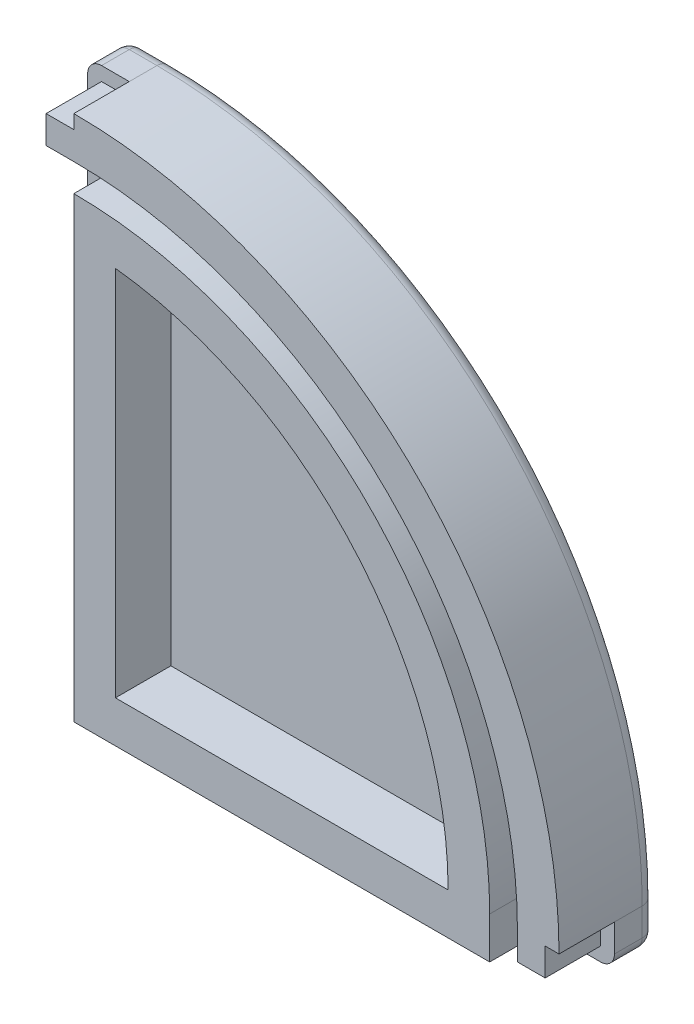
from build123d import *

# Parameters (mm, degrees)
BOSS_EXTRUDE1_DEPTH = 1.5
BOSS_EXTRUDE2_DEPTH = 2
FILETE1_R           = 0.5


with BuildPart() as part:
    # Sketch1 → Boss-Extrude1 (new body)
    with BuildSketch(Plane.XY):
        with BuildLine():
            Line((0, 0), (0, 19))
            Line((0, 19), (1.5, 19))
            ThreePointArc((1.5, 19), (13.874368671, 13.874368671), (19, 1.5))
            Line((19, 1.5), (19, 0))
            Line((19, 0), (0, 0))
        make_face()
    extrude(amount=BOSS_EXTRUDE1_DEPTH)

    # Sketch2 → Boss-Extrude2 (add)
    # profile 1 of 2: a face of its own
    with BuildSketch(Plane.XY.offset(1.5)):
        with BuildLine():
            Line((1.5, 19), (1.5, 18.5))
            Line((1.5, 18.5), (0.5, 18.5))
            Line((0.5, 18.5), (0.5, 17.5))
            Line((0.5, 17.5), (1.5, 17.5))
            ThreePointArc((1.5, 17.5), (12.813708499, 12.813708499), (17.5, 1.5))
            Line((17.5, 1.5), (17.5, 0.5))
            Line((17.5, 0.5), (18.5, 0.5))
            Line((18.5, 0.5), (18.5, 1.5))
            Line((18.5, 1.5), (19, 1.5))
            ThreePointArc((19, 1.5), (13.874368671, 13.874368671), (1.5, 19))
        make_face()
    # profile 2 of 2: a face of its own
    with BuildSketch(Plane.XY.offset(1.5)):
        with BuildLine():
            Line((1.5, 16.5), (1.5, 0))
            Line((1.5, 0), (16.5, 0))
            Line((16.5, 0), (16.5, 1.5))
            ThreePointArc((16.5, 1.5), (12.106601718, 12.106601718), (1.5, 16.5))
        make_face()
        with BuildLine():
            Line((3, 14.916407865), (3, 1.5))
            Line((3, 1.5), (15, 1.5))
            ThreePointArc((15, 1.5), (11.562305899, 10.5), (3, 14.916407865))
        make_face(mode=Mode.SUBTRACT)
    extrude(amount=BOSS_EXTRUDE2_DEPTH)

    # Filete1
    filete1_edges = [part.edges().sort_by_distance(p)[0] for p in [
        (0, 9.5, 0),
        (0.75, 19, 0),
        (13.874368671, 13.874368671, 0),
        (19, 0.75, 0),
        (9.5, 0, 0),
        (0, 19, 0.75),
        (19, 0, 0.75),
    ]]
    fillet(filete1_edges, radius=FILETE1_R)


solid = part.part
